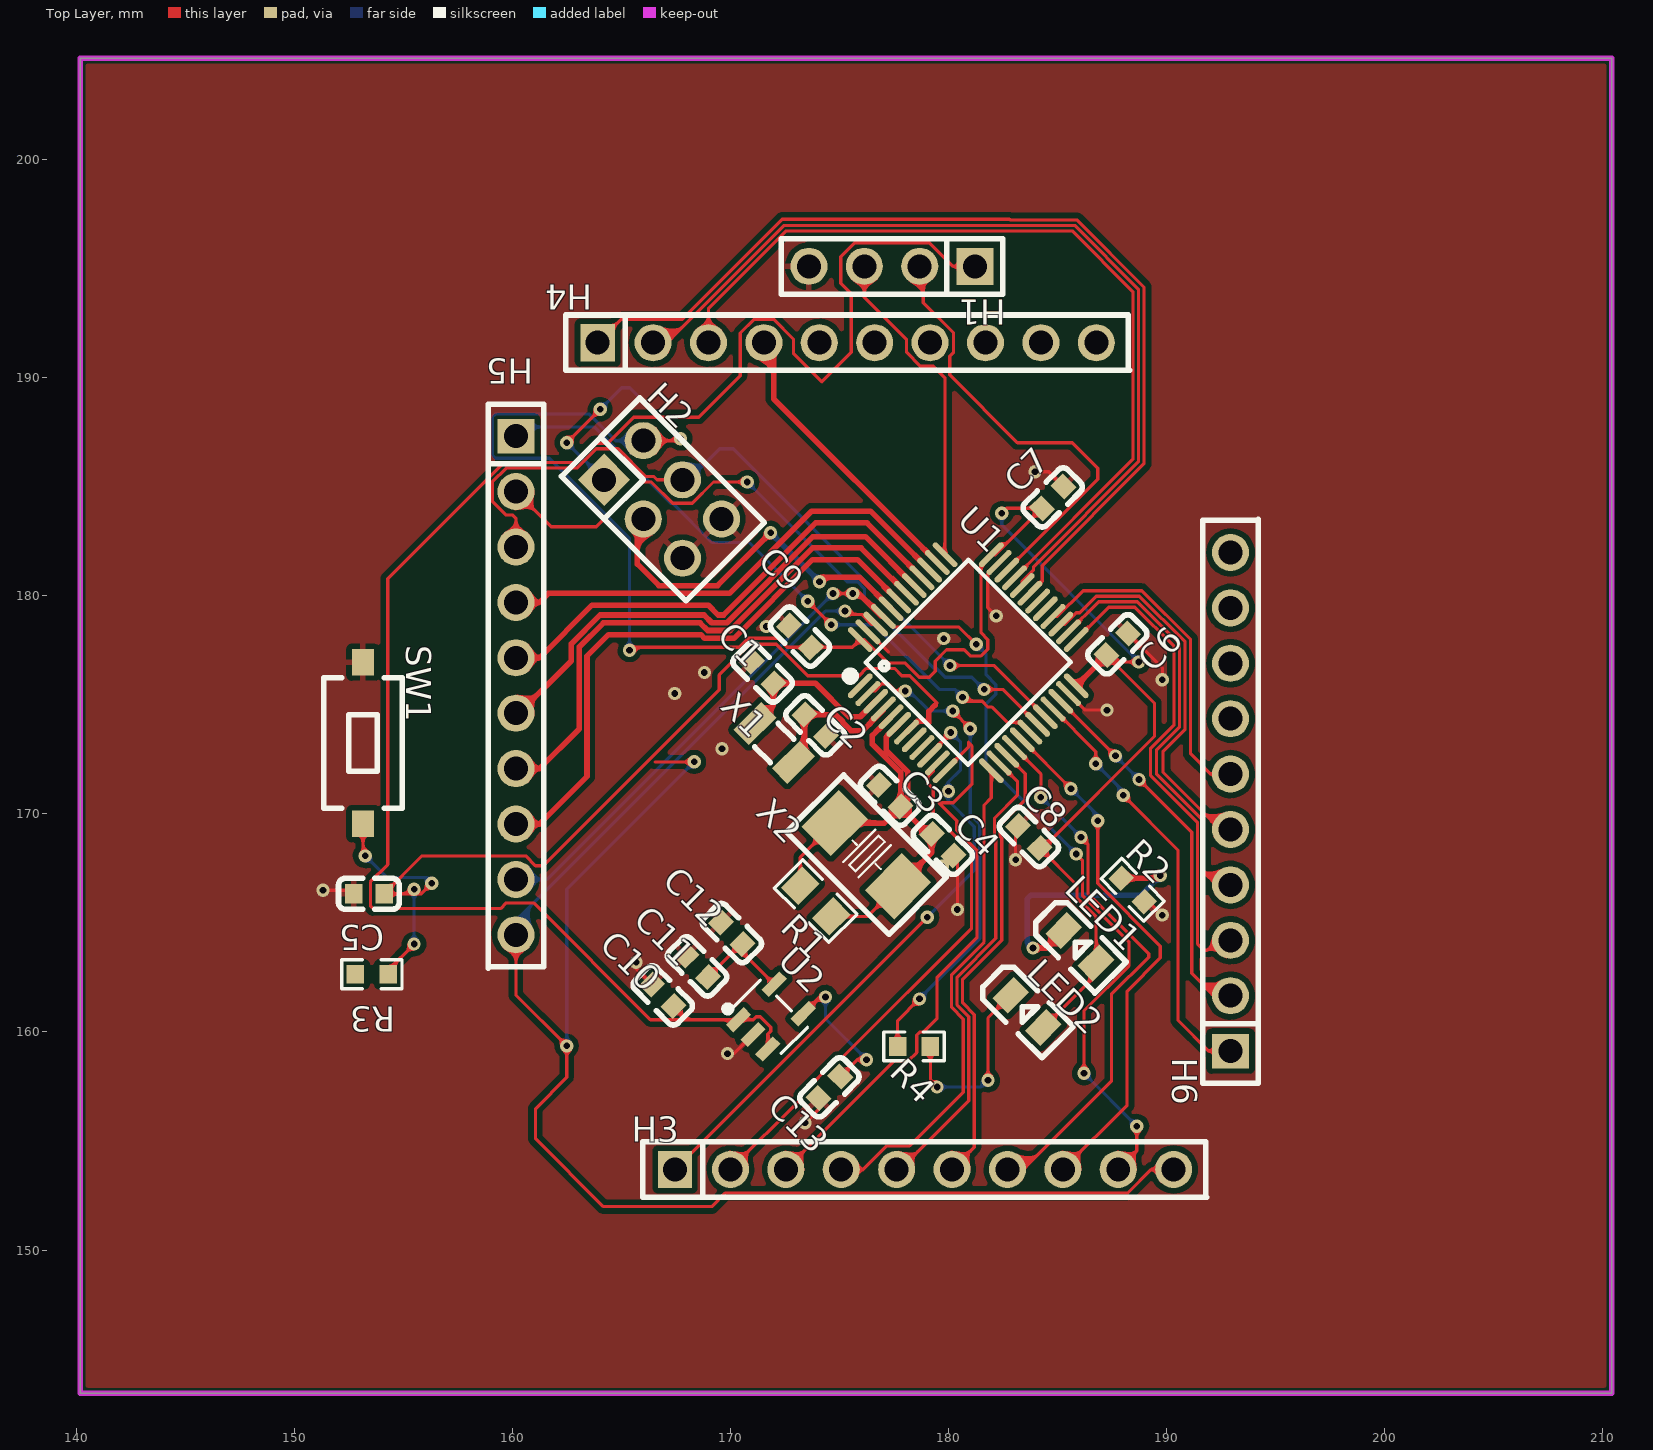
[diagram p0: Top Layer view]
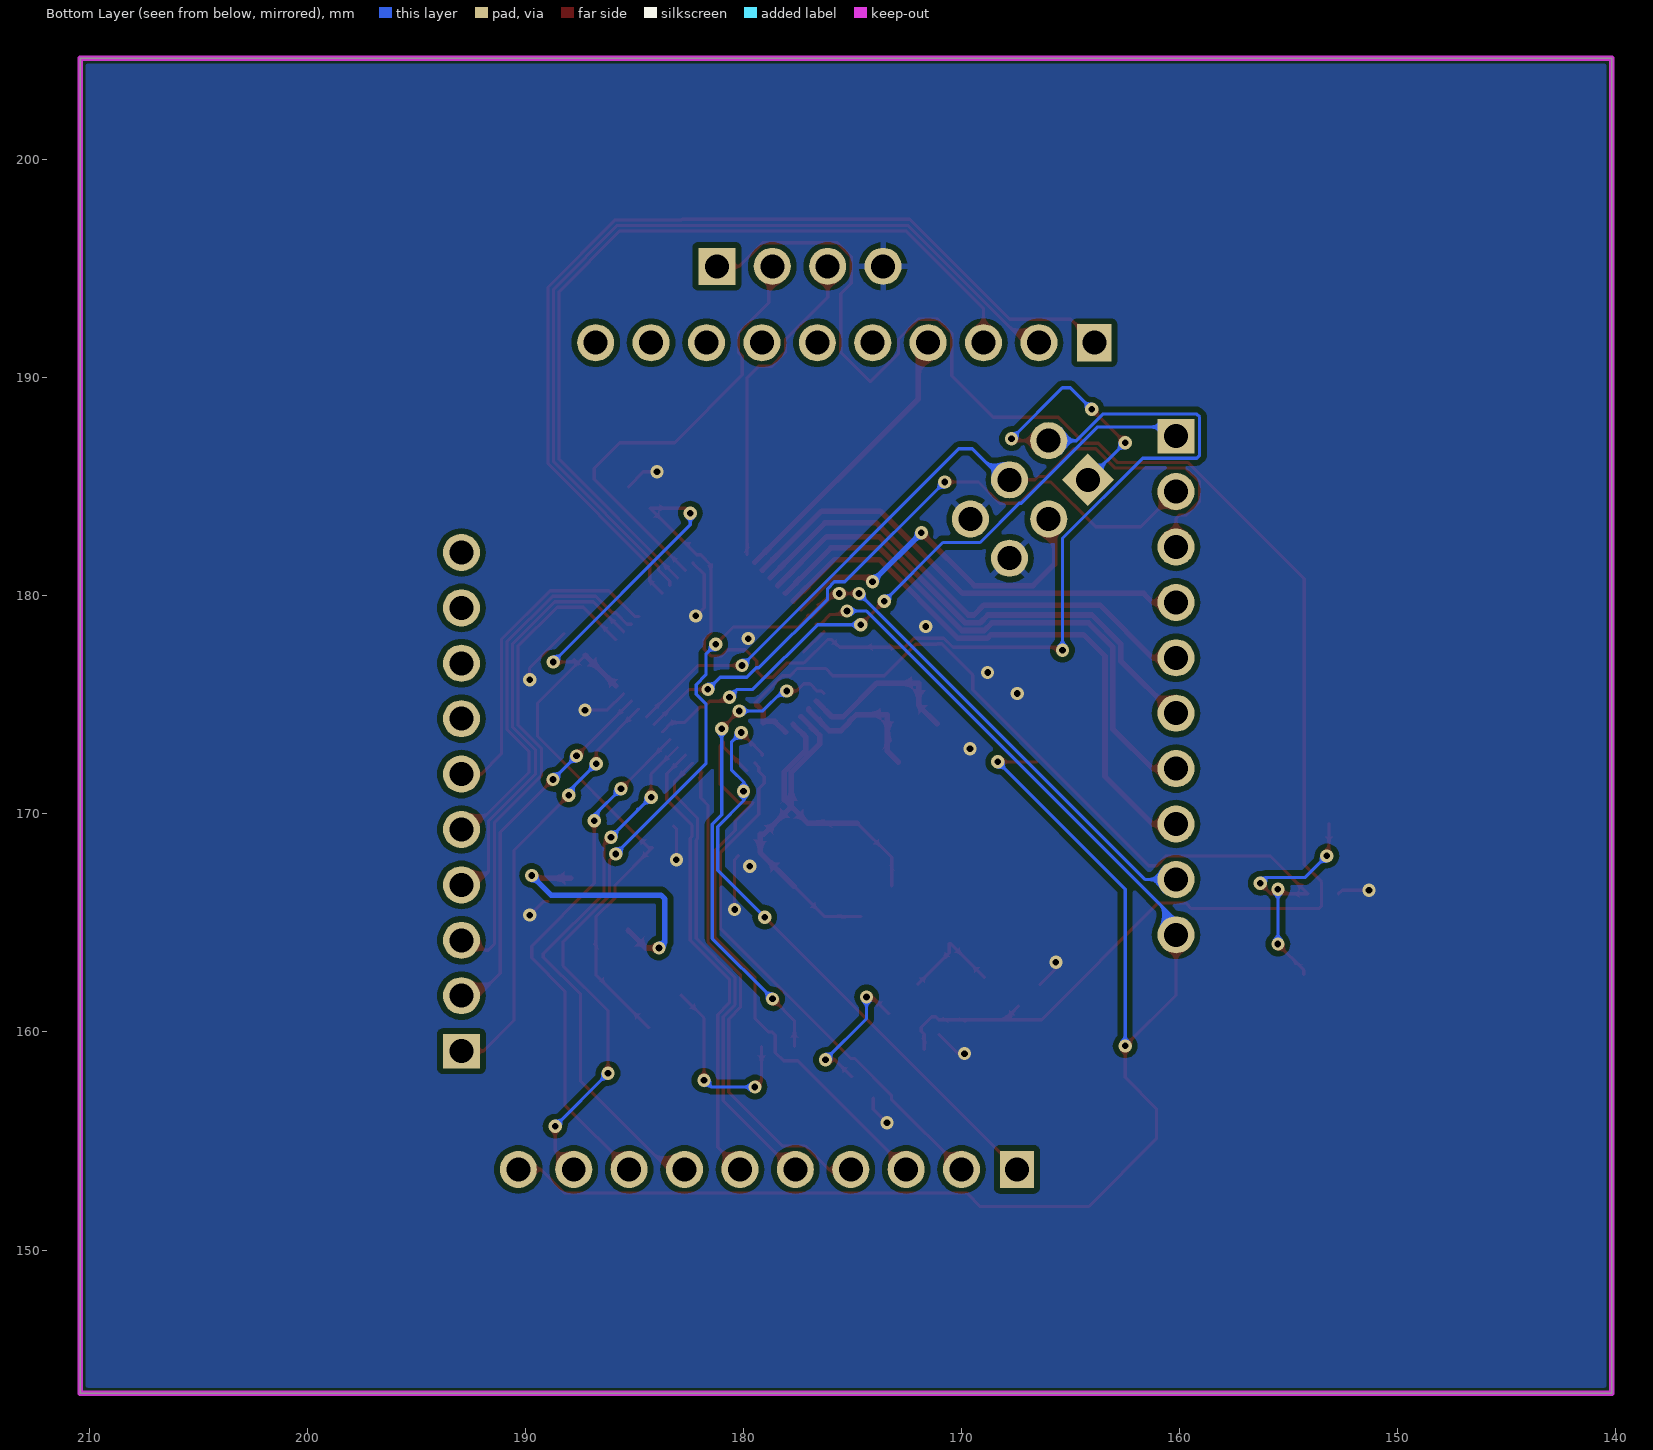
[diagram p1: Bottom Layer view, seen from below]
# Altium PCB MISC52025.pcbdoc
Units mm, origin at the board's own origin, x right, y up, seen from the top; angles counter-clockwise.
Board outline 70.23 x 61.21 mm, 2 copper layers (Top Layer, Bottom Layer), stack 1.58 mm thick; 30 components, 46 nets, 147 pads, 65 vias.

## Layer stack, top to bottom
Top Solder Mask Layer: solder mask 0.01, Dk 3.3
Top Layer: signal copper 0.035
Dielectric1: surface 1.51, FR4, Dk 4.5
Bottom Layer: signal copper 0.035
Bottom Solder Mask Layer: solder mask 0.01, Dk 3.3

## Board outline
140.182,204.647 140.182,143.433 210.413,143.433 210.413,204.647

## Design rules (kind name [scope] priority, off if disabled: settings)
BoardOutlineClearance copperThickness2oz_1 [All] p2 off: genericclearance=0.203 ignorepadtopadclearanceinfootprint=FALSE except(0: Arc-SplitContinuation Track-SplitContinuation SMDPad-SplitContinuation THPad-SplitContinuation Via-SplitContinuation Fill-SplitContinuation Region-SplitContinuation Poly-SplitContinuation Text-SplitContinuation Hole-SplitContinuation; 0.152: Arc-CutoutEdge SMDPad-CutoutEdge THPad-CutoutEdge Via-CutoutEdge Fill-CutoutEdge Region-CutoutEdge Text-CutoutEdge; 0.176: Hole-OutlineEdge Hole-CutoutEdge; 0.254: Poly-OutlineEdge Poly-CutoutEdge; 0.3: Arc-OutlineEdge Track-OutlineEdge SMDPad-OutlineEdge THPad-OutlineEdge Via-OutlineEdge Fill-OutlineEdge Region-OutlineEdge Text-OutlineEdge Track-CutoutEdge)
BoardOutlineClearance copperThickness1oz_1 [All] p4: genericclearance=0.102 ignorepadtopadclearanceinfootprint=FALSE except(0: Arc-SplitContinuation Track-SplitContinuation SMDPad-SplitContinuation THPad-SplitContinuation Via-SplitContinuation Fill-SplitContinuation Region-SplitContinuation Poly-SplitContinuation Text-SplitContinuation Hole-SplitContinuation; 0.152: SMDPad-CutoutEdge THPad-CutoutEdge Via-CutoutEdge Fill-CutoutEdge Region-CutoutEdge Text-CutoutEdge; 0.176: Hole-OutlineEdge Hole-CutoutEdge; 0.254: Poly-OutlineEdge Poly-CutoutEdge; 0.3: Arc-OutlineEdge Track-OutlineEdge SMDPad-OutlineEdge THPad-OutlineEdge Via-OutlineEdge Fill-OutlineEdge Region-OutlineEdge Text-OutlineEdge Arc-CutoutEdge Track-CutoutEdge)
Clearance copperThickness2oz [All] p1 off: gap=0.203 ignorepadtopadclearanceinfootprint=FALSE except(0.152: SMDPad-Track SMDPad-SMDPad THPad-Track SMDPad-THPad THPad-THPad Track-Via SMDPad-Via THPad-Via Via-Via Fill-Track Region-Track Fill-SMDPad Region-SMDPad Fill-THPad Region-THPad Fill-Via Region-Via Fill-Fill Fill-Region Region-Region Arc-Track Arc-SMDPad Arc-THPad Arc-Via Fill-Arc Region-Arc Arc-Arc Text-Track SMDPad-Text Text-THPad Text-Via Fill-Text Region-Text Arc-Text Text-Text; 0.176: Hole-Track Hole-SMDPad Hole-THPad Hole-Via Fill-Hole Region-Hole Hole-Arc Hole-Text; 0.254: Poly-Track Poly-SMDPad Poly-THPad Poly-Via Poly-Fill Poly-Region Poly-Poly Poly-Arc Poly-Text Poly-Hole)
Clearance copperThickness1oz [All] p3: gap=0.102 ignorepadtopadclearanceinfootprint=FALSE except(0.152: SMDPad-Track SMDPad-SMDPad THPad-Track SMDPad-THPad THPad-THPad Track-Via SMDPad-Via THPad-Via Via-Via Fill-Track Region-Track Fill-SMDPad Region-SMDPad Fill-THPad Region-THPad Fill-Via Region-Via Fill-Fill Fill-Region Region-Region Arc-Track Arc-SMDPad Arc-THPad Arc-Via Fill-Arc Region-Arc Arc-Arc Text-Track SMDPad-Text Text-THPad Text-Via Fill-Text Region-Text Arc-Text Text-Text; 0.176: Hole-Track Hole-SMDPad Hole-THPad Hole-Via Fill-Hole Region-Hole Hole-Arc Hole-Text; 0.254: Poly-Track Poly-SMDPad Poly-THPad Poly-Via Poly-Fill Poly-Region Poly-Poly Poly-Arc Poly-Text Poly-Hole)
DiffPairsRouting differentialPair [All] p1: maxlimit=0.152 minlimit=0.152 mostfreqgap=0.152 toplayer_minwidth=0.127 toplayer_prefwidth=0.254 toplayer_maxwidth=2.54 toplayer_mingap=0.152 toplayer_prefgap=0.152 toplayer_maxgap=0.152 bottomlayer_minwidth=0.127 bottomlayer_prefwidth=0.254 bottomlayer_maxwidth=2.54 bottomlayer_mingap=0.152 bottomlayer_prefgap=0.152 bottomlayer_maxgap=0.152 maxuncoupledlength=0.254
HoleToHoleClearance otherClearance [All] p1: gap=0.3 allowstackedmicrovias=TRUE
Length netLength [All] p1: minlimit=0 maxlimit=0
MatchedLengths netLengthTolerance [All] p1: tolerance=25.4
PasteMaskExpansion pasteMaskExpansion [All] p1: expansion=0
PlaneConnect innerPlane [All] p1: planeconnectstyle=Relief reliefexpansion=0.508 reliefentries=4 reliefconductorwidth=0.254 reliefairgap=0.254
PolygonConnect copperRegion [(InNet('GND'))] p1: connectstyle=Relief reliefconductorwidth=0.254 reliefentries=4 polygonreliefangle="90 Angle" airgapwidth=0.254 via.connectstyle=Relief via.reliefconductorwidth=0.254 via.reliefentries=4 via.polygonreliefangle="90 Angle" via.airgapwidth=0.254
RoutingVias viaSize [All] p1: holewidth=0.305 width=0.61 viastyle="Through Hole" minholewidth=0.3 minwidth=0.5 maxholewidth=6.3 maxwidth=10
SolderMaskExpansion solderMaskExpansion [IsVia] p1: expansion=-25.4 istentingtop=TRUE
SolderMaskExpansion solderMaskExpansion [All] p2: expansion=0.051 istentingtop=FALSE
Width copperThickness2oz_2 [All] p1 off: maxlimit=2.54 minlimit=0.203 preferedwidth=0.254
Width copperThickness1oz_2 [All] p2: maxlimit=2.54 minlimit=0.127 preferedwidth=0.254

## Components (designator, comment, footprint, x,y, rotation, side; value= is the part's Value field where it differs from the comment)
C1 "22pF" C0603 171.471,176.478 r315 top
C2 "22pF" C0603 173.895,174.053 r135 top
C3 "22pF" C0603 177.308,170.82 r315 top
C4 "22pF" C0603 179.733,168.575 r135 top
C5 "100nF" C0603 153.421,166.33 r0 top
C6 "100nF" C0603 187.735,177.767 r225 top
C7 "100nF" C0603 184.771,184.502 r225 top
C8 "100nF" C0603 183.684,168.934 r315 top
C9 "100nF" C0603 173.187,178.126 r315 top
C10 "10uF" C0603 166.901,161.672 r315 top
C11 "100nF" C0603 168.468,163.001 r315 top
C12 "1uF" C0603 170.066,164.53 r315 top
C13 "22nF" C0603 174.538,157.457 r45 top
H1 "PZ254V-11-04P" HDR-TH_4P-P2.54-V-M 177.407,195.099 r180 top
H2 "PZ254V-12-6P" HDR-TH_6P-P2.54-V-M-R2-C3-S2.54 166.901,184.412 r315 top
H3 "PH2.54-1X10P-H25" HDR-TH_10P-P2.54-V-M 178.889,153.695 r0 top
H4 "PH2.54-1X10P-H25" HDR-TH_10P-P2.54-V-M 175.342,191.596 r0 top
H5 "PH2.54-1X10P-H25" HDR-TH_10P-P2.54-V-M 160.165,175.881 r270 top
H6 "PH2.54-1X10P-H25" HDR-TH_10P-P2.54-V-M 192.929,170.55 r90 top
LED1 "HL-PSC-2012H233W(6000-7000K)" LED0805-R-RD 186.019,163.905 r315 top
LED2 "HL-PSC-2012H233W(6000-7000K)" LED0805-R-RD 183.594,160.942 r315 top
R1 "1MΩ" R0805 173.909,165.999 r315 top
R2 "510Ω" R0603 188.444,166.51 r315 top
R3 "10kΩ" R0603 153.558,162.641 r180 top
R4 "510Ω" R0603 178.414,159.332 r180 top
SW1 "TS-1101-C-W" SW-SMD_L6.0-W3.3-LS8.0_TS-1101-C-W 153.151,173.245 r270 top
U1 "STM32F103C8T6" LQFP-48_L7.0-W7.0-P0.50-LS9.0-BL 180.9,176.927 r315 top
U2 "RT9193-33GB" SOT-23-5_L3.0-W1.7-P0.95-LS2.8-BL 171.853,160.698 r315 top
X1 "32.768kHz" FC-135R_L3.2-W1.5 172.01,173.245 r135 top
X2 "8MHz" CRYSTAL-SMD_L5.0-W3.2 176.23,168.126 r135 top

## Footprints (in the part's own frame and the unit in brackets; to place one, negate y for a bottom-side part, rotate by r counter-clockwise, add the part's x,y. Pads: shape width x height; smd on the part's side, far side on the other; paste and mask are expansions set on the pad)
C0603 [mm]
  rect 0.8x0.9 smd: 1(-0.7,0) 2(0.7,0)
  silkscreen extent -1.39,-0.71 1.39,0.71
CRYSTAL-SMD_L5.0-W3.2 [mm]
  rect 1.9x2.4 smd: 1(-2.05,0) 2(2.05,0)
  silkscreen extent -3.32,-1.85 3.33,1.85
FC-135R_L3.2-W1.5 [mm]
  rect 1x1.8 smd: 1(-1.25,0) 2(1.25,0)
  silkscreen extent -0.51,-0.76 0.51,0.76
HDR-TH_4P-P2.54-V-M [mm]
  rect 1.7x1.7 hole 1.1: 1(-3.81,0)
  round 1.7 hole 1.1: 2(-1.27,0) 3(1.27,0) 4(3.81,0)
  silkscreen extent -5.08,-1.27 5.08,1.27
HDR-TH_6P-P2.54-V-M-R2-C3-S2.54 [mm]
  rect 1.7x1.7 hole 1.1: 1(-2.54,-1.27)
  round 1.7 hole 1.1: 2(-2.54,1.27) 3(0,-1.27) 4(0,1.27) 5(2.54,-1.27) 6(2.54,1.27)
  silkscreen extent -4.04,-2.54 4.04,2.54
HDR-TH_10P-P2.54-V-M [mm]
  rect 1.575x1.7 hole 1.1: 1(-11.43,0)
  round 1.7 hole 1.1: 2(-8.89,0) 3(-6.35,0) 4(-3.81,0) 5(-1.27,0) 6(1.27,0) 7(3.81,0) 8(6.35,0) 9(8.89,0) 10(11.43,0)
  silkscreen extent -12.9,-1.27 12.95,1.27
LED0805-R-RD [mm]
  rect 1x1.4 smd: 1(1.05,0) 2(-1.05,0)
  silkscreen extent -2.22,-1.04 1.99,1.01
LQFP-48_L7.0-W7.0-P0.50-LS9.0-BL [mm]
  oval 0.27x1.5 smd paste+0 mask+0.05: 1(-2.75,-4.25) 2(-2.25,-4.25) 3(-1.75,-4.25) 4(-1.25,-4.25) 5(-0.75,-4.25) 6(-0.25,-4.25) 7(0.25,-4.25) 8(0.75,-4.25) 9(1.25,-4.25) 10(1.75,-4.25) 11(2.25,-4.25) 12(2.75,-4.25) 25(2.75,4.25) 26(2.25,4.25) 27(1.75,4.25) 28(1.25,4.25) 29(0.75,4.25) 30(0.25,4.25) 31(-0.25,4.25) 32(-0.75,4.25) 33(-1.25,4.25) 34(-1.75,4.25) 35(-2.25,4.25) 36(-2.75,4.25)
  oval 1.5x0.27 smd paste+0 mask+0.05: 13(4.25,-2.75) 14(4.25,-2.25) 15(4.25,-1.75) 16(4.25,-1.25) 17(4.25,-0.75) 18(4.25,-0.25) 19(4.25,0.25) 20(4.25,0.75) 21(4.25,1.25) 22(4.25,1.75) 23(4.25,2.25) 24(4.25,2.75) 37(-4.25,2.75) 38(-4.25,2.25) 39(-4.25,1.75) 40(-4.25,1.25) 41(-4.25,0.75) 42(-4.25,0.25) 43(-4.25,-0.25) 44(-4.25,-0.75) 45(-4.25,-1.25) 46(-4.25,-1.75) 47(-4.25,-2.25) 48(-4.25,-2.75)
  silkscreen extent -3.59,-4.46 3.3,3.34
R0603 [mm]
  rect 0.806x0.864 smd paste-100 mask+0.051: 1(-0.753,0) 2(0.753,0)
  silkscreen extent -1.39,-0.66 1.39,0.66
R0805 [mm]
  rect 1.133x1.377 smd paste-100 mask+0.051: 1(-1,0) 2(1,0)
  silkscreen extent -1.76,-0.92 1.76,0.92
SOT-23-5_L3.0-W1.7-P0.95-LS2.8-BL [mm]
  rect 0.49x1.157 smd: 1(-0.95,-1.154) 2(0,-1.154) 3(0.95,-1.154)
  rect 0.49x1.175 smd: 4(0.95,1.154) 5(-0.95,1.154)
  silkscreen extent -1.8,-1.29 1.53,0.85
SW-SMD_L6.0-W3.3-LS8.0_TS-1101-C-W [mm]
  rect 1.2x1 smd: 1(-3.7,0) 2(3.7,0)
  silkscreen extent -3,-1.8 3,1.8

## Via types
v1: diameter 0.61, hole 0.305, Top Layer to Bottom Layer, 65 vias

## Nets (pads, with @x,y where several pads share a name; then routed paths per layer and width w, separated by ;. In a path a pad name is that pad's centre, name@x,y a point inside that pad or via, vN(x,y) a via of type N, cw(c..) or ccw(c..) an arc to the next point about the centre after c; other vN are vias at no path point)
$1N2: LED1.2 R2.1 | length 12.5
  Top Layer w0.254: v1(183.873,163.847) 184.475,163.847 LED1.2 ; R2.1 189.583,167.042 v1(189.71,167.17)
  Bottom Layer w0.254: v1(183.873,163.847) 183.604,164.117 183.604,166.092 183.783,166.272 188.812,166.272 v1(189.71,167.17)
$1N4: LED2.2 R4.1 | length 8.8
  Top Layer w0.15: R4.1 179.168,157.776 v1(179.473,157.471) ; v1(181.808,157.778) 181.808,160.641 LED2.2
  Bottom Layer w0.15: v1(179.473,157.471) 181.449,157.471 181.755,157.778 v1(181.808,157.778)
$1N5: R4.2 U1.2 | length 22
  Top Layer w0.15: U1.2 176.419,175.628 176.614,175.628 176.942,175.956 177.242,175.956 177.571,175.628 v1(178.02,175.628) ; R4.2 177.661,160.509 v1(178.665,161.512) ; v1(180.191,174.713) v1(181,173.905)
  Bottom Layer w0.15: v1(178.02,175.628) 178.051,175.597 178.231,175.597 179.114,174.713 v1(180.191,174.713) ; v1(178.665,161.512) 181.431,164.279 181.431,169.519 181,169.951 v1(181,173.905)
$1N7: C1.2 U1.3 X1.2 | length 7.8
  Top Layer w0.254: X1.2 171.966,174.969 C1.2 173.893,175.983 175.432,174.444 175.942,174.444 U1.3
$1N12: C3.2 C4.2 R1.1 R1.2 U1.5 U1.6 X2.1 X2.2 | length 25.1
  Top Layer w0.15: R1.1 173.202,167.997 X2.2 ; R1.2 176.295,165.292 X2.1
  Top Layer w0.254: X2.2 177.053,169.576 C3.2 ; U1.5 176.509,173.597 176.509,173.187 177.803,171.893 C3.2 ; X2.1 179.238,168.234 C4.2 179.058,169.07 C3.2 ; U1.6 177.138,173.518 177.138,172.917 178.126,171.93 178.126,170.648 C3.2
$1N13: C2.2 U1.4 X1.1 | length 6.8
  Top Layer w0.254: X1.1 173.401,172.868 C2.2 174.824,174.548 175.147,174.225 175.147,174.19 175.522,173.815 176.075,173.815 177.011,174.751 U1.4
$1N15: C5.2 R3.1 SW1.2 U1.7 | length 46.6
  Top Layer w0.15: SW1.2 153.151,168.168 v1(153.251,168.068) ; R3.1 154.312,162.843 v1(155.496,164.027) ; v1(155.496,166.541) v1@155.284,166.33 ; v1(156.304,166.811) 155.823,166.33 v1@155.284,166.33 ; 179.473,175.073 178.216,176.33 177.854,176.33 177.52,176.663 176.235,176.663 175.902,176.33 173.546,176.33 172.109,177.767 171.139,177.767 171.105,177.801 170.917,177.801 169.483,176.367 169.483,175.679 161.423,167.619 161.06,167.619 160.611,168.068 155.858,168.068 C5.2 v1@155.284,166.33
  Top Layer w0.254: U1.7 178.567,174.24 179.032,174.24 179.097,174.175 179.097,174.697 179.383,174.983
  Bottom Layer w0.15: v1(153.251,168.068) 154.238,167.08 156.034,167.08 v1(156.304,166.811) ; v1(155.496,164.027) v1(155.496,166.541)
$1N18: H1.2 U1.34 | length 20.7
  Top Layer w0.15: H1.2 178.844,194.932 178.844,193.427 180.229,192.042 180.229,191.15 180.049,190.97 180.049,190.122 183.155,187.016 185.669,187.016 186.837,185.849 186.837,185.338 U1.34
$1N19: H1.3 U1.37 | length 15.1
  Top Layer w0.15: H1.3 176.137,193.675 178.075,191.737 178.075,191.15 178.706,190.519 179.293,190.519 179.84,189.972 U1.37
$1N32: C13.2 U2.4 | length 6.5
  Top Layer w0.15: U2.4 174.101,161.602 v1(174.354,161.602) ; C13.2 175.809,158.729 v1(176.24,158.729)
  Bottom Layer w0.15: v1(174.354,161.602) 174.354,160.614 v1(176.24,158.729)
+3,3V: R3.2
+3.3V: C6.2 C7.2 C8.2 C9.2 H2.1 H2.2 LED1.1 LED2.1 U1.24 U1.36 U1.48 | length 97
  Top Layer w0.15: v1(162.5,187.016) v1(164.027,188.543) ; v1(165.374,177.497) 165.508,177.631 170.391,177.631 170.813,178.053 172.179,178.053 172.601,177.631 C9.2 175.594,177.631 U1.48 176.146,177.987 177.218,176.915 177.993,176.915 178.65,176.257 179.115,176.257 179.389,176.531 179.389,177 179.904,177.515 180.71,177.515 180.99,177.235 181.489,177.235 181.801,177.546 181.801,177.987 181.489,178.299 181.489,181.405 U1.36 182.146,181.877 C7.2 182.66,184.007 v1(182.436,183.783) ; H2.2 167.619,187.106 v1(167.709,187.196) ; LED2.1 186.762,162.624 LED1.1 186.762,165.275 185.884,166.153 185.884,166.735 C8.2 184.334,168.439 189.441,173.546 189.441,175.07 C6.2@187.553,176.958 ; C6.2 C6.2@187.553,176.958 ; v1(188.723,176.958) C6.2@187.553,176.958
  Top Layer w0.254: U1.24 187.24,177.256 C6.2
  Bottom Layer w0.15: v1(162.5,187.016) H2.1 ; v1(164.027,188.543) 165.015,189.531 165.374,189.531 v1(167.709,187.196) ; v1(165.374,177.497) 165.374,182.62 161.697,186.296 159.221,186.296 159.088,186.429 159.088,188.192 159.221,188.325 163.526,188.325 164.745,187.106 H2.2 ; v1(182.436,183.783) 182.436,183.245 v1(188.723,176.958)
+5V: C10.2 H1.1 U2.1 U2.3 | length 79.2
  Top Layer w0.15: C10.2 168.019,160.554 ; U2.3 171.709,159.886 171.847,160.024 171.847,160.212 171.367,160.692 171.179,160.692 171.042,160.554 U2.1 168.019,160.554 ; H1.1 180.201,195.099 179.124,196.176 175.691,196.176 175.06,195.545 175.06,194.318 175.535,193.843 175.535,191.15 174.192,189.807 172.885,191.114 172.885,191.766 171.978,192.673 171.086,192.673 170.455,192.042 170.455,190.087 168.552,188.183 165.556,188.183 164.364,186.991 163.735,186.991 162.844,186.1 159.615,186.1 154.291,180.776 154.291,167.671 153.494,166.874 153.494,165.786 153.627,165.653 159.459,165.653 159.719,165.914 160.973,165.914 166.332,160.554 168.019,160.554
BOOT0: H2.3 U1.44 | length 16.8
  Top Layer w0.254: H2.3 165.733,183.245 165.733,181.449 166.721,180.461 169.415,180.461 v1(171.84,182.885) ; v1(174.085,180.64) 174.297,180.853 175.913,180.853 U1.44
  Bottom Layer w0.254: v1(171.84,182.885) v1(174.085,180.64)
GND: C1.1 C2.1 C3.1 C4.1 C5.1 C6.1 C7.1 C8.1 C9.1 C10.1 C11.1 C12.1 C13.1 H1.4 H2.5 H2.6 R2.2 SW1.1 U1.23 U1.35 U1.47 U2.2 | length 21.5
  Top Layer w0.15: v1(151.322,166.498) 152.552,166.498 C5.1 ; v1(165.673,163.196) 165.673,162.9 C10.1 ; v1(169.864,159.005) 170.161,159.005 U2.2 ; v1(173.42,155.83) 174.043,156.454 C13.1 ; U1.47 177.225,177.42 177.23,177.42 ; C4.1 180.405,167.903 v1(180.405,165.609) ; v1(182.183,179.071) 181.802,179.452 181.802,180.976 182.314,181.489 U1.35 ; v1(183.072,167.895) 183.072,169.312 C8.1 ; v1(183.961,185.675) 184.588,185.675 C7.1 ; U1.23 186.255,174.753 v1(187.263,174.753) ; C6.1 189.803,176.688 v1(189.803,176.15) ; R2.2 189.181,165.977 v1(189.803,165.355)
  other v1: 179.712,167.592 169.61,172.975 167.451,175.515 168.806,176.478 179.778,178.031 171.642,178.585
PA0: H3.1 U1.10 | length 28.1
  Top Layer w0.15: H3.1 v1(179.023,165.259) ; U1.10 179.132,172.756 v1(180.102,173.726)
  Bottom Layer w0.15: v1(179.023,165.259) 181.179,167.415 181.179,169.415 179.974,170.62 v1@179.974,171.032 ; v1(179.995,171.032) v1@179.974,171.032 ; v1(180.102,173.726) 180.551,173.277 180.551,172.019 179.974,171.443 v1@179.974,171.032
PA1: H3.2 U1.11 | length 24.3
  Top Layer w0.15: H3.2 173.215,156.912 173.215,157.092 174.904,158.781 175.084,158.781 181.056,164.752 181.056,168.21 179.293,169.972 179.293,171.142 179.043,171.392 179.043,171.692 179.293,171.943 179.293,172.138 U1.11
PA2: H3.3 U1.12 | length 27.2
  Top Layer w0.15: H3.3 177.516,158.673 178.158,158.673 178.538,159.052 178.538,159.858 178.671,159.991 178.834,159.991 179.473,160.629 179.473,162.5 181.308,164.335 181.308,168.314 180.371,169.251 180.371,169.684 179.563,170.493 179.57,170.5 180.216,170.5 181.072,171.356 181.072,173.112 180.91,173.274 180.91,173.047 U1.12
PA3: H3.4 U1.13 | length 22.8
  Top Layer w0.15: H3.4 176.096,153.695 177.173,154.772 178.21,154.772 180.675,157.237 180.675,160.585 180.136,161.124 180.136,162.625 181.628,164.117 181.628,170.403 181.961,170.735 U1.13
PA4: H3.5 U1.14 | length 21.9
  Top Layer w0.15: H3.5 177.784,153.695 180.927,156.839 180.927,160.69 180.388,161.228 180.388,162.515 182.167,164.293 182.167,168.789 182.109,168.847 182.109,169.806 183.155,170.852 183.155,171.49 U1.14
PA5: H3.6 U1.15 | length 21.2
  Top Layer w0.15: H3.6 181.179,154.715 181.179,160.794 180.64,161.333 180.64,162.41 182.436,164.207 182.436,168.876 182.361,168.952 182.361,169.488 183.514,170.641 183.514,171.838 U1.15
PA6: H3.7 U1.16 | length 25.1
  Top Layer w0.15: H3.7 183.42,153.695 187.465,157.741 187.465,161.722 189.172,163.428 189.172,163.578 186.388,166.362 186.388,168.607 v1(186.073,168.921) ; U1.16 184.232,171.827 v1(184.232,170.762)
  Bottom Layer w0.15: v1(184.232,170.762) 184.771,170.223 ; 184.861,170.223 184.771,170.223 ; v1(186.073,168.921) 184.771,170.223
PA7: H3.8 U1.17 | length 24.2
  Top Layer w0.15: U1.17 v1(185.612,171.154) ; H3.8 188.184,156.64 188.184,161.872 189.71,163.398 189.71,163.937 186.837,166.811 v1(186.837,169.684)
  Bottom Layer w0.15: v1(185.612,171.154) 186.837,169.929 v1(186.837,169.684)
PA8: U1.29
PA9: U1.30
PA10: H4.1 U1.31 | length 44.9
  Top Layer w0.15: H4.1 164.99,192.674 167.799,192.674 172.379,197.254 182.796,197.254 182.825,197.224 185.883,197.224 188.957,194.151 188.957,186.039 184.3,181.381 184.3,180.68 U1.31
PA11: H4.2 U1.32 | length 41.5
  Top Layer w0.15: H4.2 167.08,191.596 168.427,192.943 168.43,192.943 172.459,196.972 185.779,196.972 188.705,194.046 188.705,186.143 183.895,181.333 183.895,181.178 183.375,180.657 U1.32
PA12: H4.3 U1.33 | length 39
  Top Layer w0.15: H4.3 168.992,193.149 172.563,196.72 185.675,196.72 188.453,193.942 188.453,186.248 U1.33
PA15: H4.4 U1.38 | length 13.4
  Top Layer w0.254: H4.4 171.981,191.147 171.981,189.028 U1.38
PB0: H5.1 U1.18 | length 29.5
  Top Layer w0.15: v1(173.546,179.742) v1(174.624,178.665) ; v1(180.64,175.342) 180.82,175.162 181.538,175.162 181.808,174.893 181.994,174.893 182.699,174.188 183.285,174.188 U1.18
  Bottom Layer w0.15: H5.1 160.589,187.735 163.757,187.735 167.26,184.232 167.353,184.232 169.149,182.437 170.851,182.437 v1(173.546,179.742) ; v1(174.624,178.665) 176.599,178.665 179.563,175.701 180.281,175.701 v1(180.64,175.342)
PB1: H5.2 U1.19 | length 31.1
  Top Layer w0.15: H5.2 161.781,183.155 163.847,183.155 165.904,185.211 166.374,185.211 167.353,184.233 168.245,184.233 169.223,185.211 v1(170.771,185.211) ; v1(181.628,175.701) 182.479,175.701 U1.19
  Bottom Layer w0.15: v1(170.771,185.211) 175.349,180.634 175.832,180.634 176.143,180.322 176.143,179.839 179.293,176.689 179.419,176.689 179.845,176.263 181.067,176.263 v1(181.628,175.701)
PB2: H2.4 H5.3 U1.20 | length 35.9
  Top Layer w0.15: H5.3 160.165,183.548 160.02,183.694 159.719,183.694 159.088,184.325 159.088,185.217 159.719,185.848 162.948,185.848 163.84,186.739 164.846,186.739 166.122,185.463 166.479,185.463 166.632,185.31 H2.4 ; v1(180.065,176.795) 182.093,176.795 U1.20
  Bottom Layer w0.15: H2.4 168.078,185.31 169.505,186.737 170.123,186.737 v1(180.065,176.795)
PB3: H5.4 U1.39 | length 21.8
  Top Layer w0.254: H5.4 161.243,179.691 161.654,180.102 169.954,180.102 173.726,183.873 176.42,183.873 179.124,181.169 U1.39
PB4: H5.5 U1.40 | length 22.6
  Top Layer w0.254: H5.5 161.243,177.151 163.655,179.563 168.981,179.563 169.43,179.114 169.684,179.114 173.905,183.334 176.26,183.334 U1.40
PB5: H5.6 U1.41 | length 23.3
  Top Layer w0.254: H5.6 160.3,174.611 162.7,177.011 162.7,177.786 164.027,179.114 168.786,179.114 169.142,178.758 169.832,178.758 173.78,182.706 176.182,182.706 U1.41
PB6: H5.7 U1.42 | length 25.5
  Top Layer w0.254: H5.7 161.243,172.071 163.066,173.894 163.066,177.65 164.171,178.755 168.607,178.755 168.96,178.402 169.979,178.402 173.766,182.188 175.992,182.188 U1.42
PB7: H5.8 U1.43 | length 26.7
  Top Layer w0.254: H5.8 161.243,169.531 163.422,171.71 163.422,177.228 164.41,178.216 168.642,178.216 168.812,178.046 170.158,178.046 173.768,181.655 175.818,181.655 U1.43
PB8: H3.9 H5.9 U1.45 | length 57.1
  Top Layer w0.15: v1(174.704,180.102) v1(175.611,180.102) ; U1.45 177.496,178.563 180.472,178.563 v1(181.269,177.767) ; v1(185.849,168.158) 186.136,167.871 186.136,166.257 188.274,164.12 188.274,163.039 186.208,160.974 v1(186.208,158.1) ; H3.9 188.633,154.549 v1(188.633,155.675)
  Top Layer w0.254: v1(175.611,180.102) 175.881,180.102 176.934,179.048 U1.45
  Bottom Layer w0.15: H5.9 161.594,166.991 v1(174.704,180.102) ; v1(181.269,177.767) 181.718,177.318 181.718,176.364 182.16,175.922 182.16,175.481 181.718,175.039 181.718,172.289 v1(185.849,168.158) ; v1(186.208,158.1) v1(188.633,155.675)
PB9: H3.10 H5.10 U1.46 | length 82.7
  Top Layer w0.15: H5.10 160.165,161.692 v1(162.5,159.357) 162.5,157.92 161.063,156.483 161.063,155.107 164.177,151.993 169.146,151.993 169.77,152.618 188.225,152.618 189.302,153.695 H3.10 ; 166.539,172.379 v1(168.337,172.379) ; v1(175.252,179.293) 175.408,179.138 176.019,179.138 176.462,178.694 U1.46
  Bottom Layer w0.15: H5.10 160.165,165.105 174.354,179.293 175.008,179.293 v1(175.252,179.293) ; v1(162.5,159.357) 162.5,166.541 v1(168.337,172.379)
PB10: H6.1 U1.21 | length 19.6
  Top Layer w0.15: U1.21 186.747,172.848 v1(186.747,172.289) ; v1(188.004,170.852) 190.519,168.337 190.519,160.525 191.923,159.12 H6.1
  Bottom Layer w0.15: v1(186.747,172.289) 188.004,171.032 v1(188.004,170.852)
PB11: H6.2 U1.22 | length 17.2
  Top Layer w0.15: U1.22 v1(187.649,172.652) ; v1(188.727,171.575) 191.147,169.155 191.147,162.68 192.167,161.66 H6.2
  Bottom Layer w0.15: v1(187.649,172.652) v1(188.727,171.575)
PB12: H6.3 U1.25 | length 22.7
  Top Layer w0.15: U1.25 187.335,179.473 188.543,179.473 190.339,177.677 190.339,174.085 189.261,173.007 189.261,171.75 191.417,169.595 191.417,164.027 191.701,163.743 191.851,163.743 191.882,163.774 192.503,163.774 H6.3
PB13: H6.4 U1.26 | length 19.7
  Top Layer w0.15: U1.26 186.88,179.725 188.647,179.725 190.591,177.781 190.591,173.98 189.531,172.92 189.531,171.84 191.686,169.684 191.686,167.35 192.296,166.74 H6.4
PB14: H6.5 U1.27 | length 17.7
  Top Layer w0.15: U1.27 185.338,178.694 185.858,179.215 186.014,179.215 186.776,179.977 188.752,179.977 190.843,177.886 190.843,173.876 189.835,172.868 189.835,171.892 192.447,169.28 H6.5
PB15: H6.6 U1.28 | length 15.2
  Top Layer w0.15: U1.28 184.984,179.048 186.165,180.229 188.856,180.229 191.095,177.99 191.095,172.742 192.017,171.82 H6.6
VCC: C11.2 C12.2 U2.5 | length 4.7
  Top Layer w0.15: C11.2 170.493,164.035 C12.2 170.561,163.622 U2.5
pads on no net: H4.5 H4.6 H4.7 H4.8 H4.9 H4.10 H6.7 H6.8 H6.9 H6.10 U1.1 U1.8 U1.9

## Polygon pours and split planes (outlines as drawn)
GND on Bottom Layer (solid, remove dead copper, pour order 2): 177.497,269.904 85.988,178.395 179.653,84.731 271.161,176.24
GND on Top Layer (solid, remove dead copper, pour order 0): 174.803,284.991 76.2,186.388 186.388,76.2 284.991,174.803

## Keep-outs
Board Outline Layer:
  the board outline again, w0.254

## Other copper
Top Layer:
  drawing of 165 lines, arcs and shapes, not listed
Bottom Layer:
  region net BOOT0: 173.701,180.844 173.881,181.024 173.92,180.997 173.977,180.973 174.042,180.954 174.104,180.945 173.78,180.621 173.771,180.684 173.752,180.749 173.728,180.806
  region net BOOT0: 172.223,182.682 172.044,182.502 172.005,182.528 171.948,182.553 171.883,182.572 171.821,182.581 172.144,182.905 172.154,182.842 172.172,182.777 172.197,182.72
  region net PB8: 174.464,179.755 174.358,179.861 174.371,179.893 174.383,179.954 174.4,180.121 174.723,179.797 174.557,179.78 174.496,179.768
  region net PB8: 161.323,167.066 161.323,166.916 161.278,166.911 161.234,166.896 161.19,166.873 161.147,166.843 161.104,166.807 161.062,166.766 160.982,166.675 160.907,166.579 160.839,166.487 160.779,166.409 160.728,166.353 160.728,167.628 160.779,167.573 160.839,167.495 160.907,167.403 160.982,167.306 161.062,167.215 161.104,167.174 161.147,167.138 161.19,167.108 161.234,167.086 161.278,167.071
  region net PB9: 174.837,179.218 174.837,179.368 174.869,179.382 174.921,179.416 175.05,179.522 175.05,179.065 174.921,179.17 174.869,179.205
  region net PB9: 160.295,165.34 160.891,165.724 160.863,165.688 160.84,165.645 160.823,165.595 160.811,165.54 160.803,165.481 160.8,165.419 160.804,165.289 160.82,165.16 160.845,165.041 160.875,164.94 160.906,164.867 159.659,165.134 159.682,165.147 159.711,165.159 159.78,165.176 159.954,165.204 160.048,165.222 160.14,165.248 160.183,165.265 160.224,165.286 160.261,165.311
  region net PB11: 187.996,172.412 187.89,172.306 187.858,172.319 187.797,172.331 187.63,172.348 187.954,172.672 187.971,172.505 187.983,172.444
  region net PB11: 188.38,171.815 188.486,171.921 188.519,171.908 188.58,171.896 188.746,171.879 188.423,171.556 188.406,171.722 188.394,171.783
  region net PB10: 187.094,172.048 186.988,171.942 186.955,171.956 186.894,171.967 186.728,171.984 187.051,172.308 187.068,172.141 187.08,172.08
  region net PB10: 187.693,171.237 187.934,171.208 187.959,171.188 187.987,171.172 188.048,171.15 188.106,171.135 188.148,171.121 187.719,170.961 187.73,170.997 187.737,171.036 187.739,171.075 187.737,171.115 187.731,171.152 187.722,171.186 187.709,171.215
  region net PB2: 179.719,177.035 179.825,177.141 179.857,177.128 179.918,177.116 180.085,177.099 179.761,176.776 179.744,176.942 179.732,177.003
  region net PB2: 168.798,186.136 168.694,185.82 168.666,185.785 168.644,185.745 168.628,185.7 168.616,185.651 168.609,185.599 168.606,185.544 168.606,185.432 168.619,185.218 168.621,185.129 168.618,185.092 168.611,185.061 167.944,186.148 168.125,186.11 168.244,186.087 168.371,186.067 168.498,186.058 168.559,186.058 168.617,186.062 168.671,186.072 168.719,186.087 168.762,186.108
  region net PB1: 181.282,175.942 181.388,176.048 181.42,176.034 181.481,176.023 181.647,176.006 181.324,175.682 181.307,175.849 181.295,175.91
  region net PB1: 171.118,184.971 171.012,184.865 170.98,184.878 170.918,184.89 170.752,184.907 171.075,185.23 171.092,185.064 171.104,185.003
  region net PB0: 180.294,175.583 180.4,175.689 180.432,175.675 180.493,175.663 180.659,175.646 180.336,175.323 180.319,175.489 180.307,175.55
  region net PB0: 175.039,178.74 175.039,178.59 175.007,178.577 174.955,178.542 174.825,178.436 174.825,178.893 174.955,178.788 175.007,178.753
  region net PB0: 173.199,179.983 173.305,180.089 173.338,180.076 173.399,180.064 173.565,180.047 173.242,179.723 173.225,179.89 173.213,179.951
  region net PB0: 161.24,187.81 161.24,187.66 161.176,187.652 161.115,187.63 161.06,187.594 161.015,187.547 161.015,187.922 161.06,187.875 161.115,187.839 161.176,187.817 161.24,187.81
  region net PA7: 185.959,170.913 185.853,170.807 185.821,170.821 185.759,170.833 185.593,170.85 185.917,171.173 185.933,171.007 185.945,170.945
  region net PA7: 186.546,170.114 186.836,170.037 186.86,170.015 186.886,169.997 186.94,169.968 186.99,169.945 187.025,169.924 186.575,169.842 186.59,169.873 186.598,169.908 186.602,169.945 186.6,169.984 186.594,170.021 186.582,170.057 186.566,170.088
  region net PA6: 184.579,170.522 184.473,170.415 184.441,170.429 184.38,170.441 184.213,170.458 184.537,170.781 184.554,170.615 184.566,170.554
  region net PA6: 185.727,169.162 185.833,169.268 185.865,169.254 185.926,169.242 186.093,169.226 185.769,168.902 185.752,169.068 185.74,169.13
  region net $1N5: 181.075,173.49 180.925,173.49 180.911,173.522 180.877,173.574 180.771,173.703 181.228,173.703 181.123,173.574 181.088,173.522
  region net $1N5: 178.905,161.859 179.011,161.753 178.998,161.721 178.986,161.66 178.969,161.493 178.646,161.817 178.812,161.834 178.873,161.846
  region net PB8: 185.502,168.398 185.608,168.504 185.64,168.491 185.702,168.479 185.868,168.462 185.545,168.139 185.528,168.305 185.516,168.366
  region net PB8: 181.616,177.526 181.51,177.42 181.477,177.433 181.416,177.445 181.25,177.462 181.573,177.786 181.59,177.619 181.602,177.558
  region net PB8: 188.286,155.916 188.392,156.022 188.424,156.008 188.486,155.997 188.652,155.98 188.328,155.656 188.312,155.823 188.3,155.884
  region net PB8: 186.555,157.859 186.449,157.753 186.417,157.767 186.355,157.779 186.189,157.796 186.513,158.119 186.529,157.953 186.541,157.891
  region net $1N32: 175.893,158.969 175.999,159.075 176.032,159.062 176.093,159.05 176.259,159.033 175.936,158.709 175.919,158.876 175.907,158.937
  region net $1N32: 174.429,161.187 174.279,161.187 174.266,161.219 174.231,161.271 174.125,161.4 174.583,161.4 174.477,161.271 174.442,161.219
  region net $1N4: 179.888,157.546 179.888,157.396 179.856,157.383 179.804,157.348 179.675,157.243 179.675,157.7 179.804,157.594 179.856,157.56
  region net $1N4: 181.522,157.439 181.456,157.584 181.468,157.614 181.48,157.67 181.508,157.834 181.789,157.473 181.705,157.474 181.623,157.467 181.558,157.455 181.536,157.447
  region net PB9: 162.425,159.772 162.575,159.772 162.588,159.74 162.623,159.688 162.729,159.559 162.272,159.559 162.377,159.688 162.412,159.74
  region net PB9: 168.097,172.032 167.991,172.138 168.004,172.17 168.016,172.231 168.033,172.398 168.357,172.074 168.19,172.057 168.129,172.045
  region net PA0: 180.448,173.485 180.342,173.379 180.31,173.392 180.249,173.404 180.082,173.421 180.406,173.745 180.423,173.578 180.435,173.517
  region net PA0: 179.899,171.43 180.049,171.443 180.052,171.43 180.063,171.413 180.099,171.366 180.209,171.249 179.753,171.217 179.853,171.349 179.886,171.399
  region net PA0: 180.049,170.62 179.899,170.633 179.886,170.664 179.853,170.714 179.753,170.846 180.209,170.814 180.099,170.697 180.063,170.65 180.052,170.633
  region net $1N2: 189.507,166.787 189.327,166.966 189.353,167.005 189.378,167.062 189.397,167.127 189.406,167.189 189.73,166.866 189.667,166.856 189.602,166.837 189.545,166.813
  region net $1N2: 183.514,164.027 183.694,164.207 183.723,164.189 183.773,164.172 183.832,164.159 183.892,164.152 183.569,163.828 183.561,163.888 183.548,163.948 183.531,163.997
  region net $1N15: 155.571,166.126 155.421,166.126 155.407,166.158 155.373,166.21 155.267,166.34 155.724,166.34 155.619,166.21 155.584,166.158
  region net $1N15: 155.421,164.442 155.571,164.442 155.584,164.41 155.619,164.358 155.724,164.229 155.267,164.229 155.373,164.358 155.407,164.41
  region net $1N15: 153.597,167.827 153.491,167.721 153.459,167.735 153.398,167.747 153.231,167.764 153.555,168.087 153.572,167.921 153.584,167.86
  region net $1N15: 155.981,167.027 156.088,167.133 156.098,167.128 156.115,167.124 156.168,167.121 156.323,167.115 155.999,166.792 155.994,166.947 155.99,167 155.987,167.017
  region net $1N5: 179.776,174.638 179.776,174.788 179.808,174.802 179.86,174.836 179.99,174.942 179.99,174.485 179.86,174.59 179.808,174.625
  region net $1N5: 178.376,175.557 178.405,175.316 178.383,175.333 178.354,175.346 178.32,175.355 178.283,175.361 178.243,175.362 178.203,175.36 178.165,175.354 178.129,175.343 178.289,175.772 178.303,175.73 178.318,175.672 178.34,175.61 178.356,175.582
  region net +3.3V: 188.376,177.199 188.482,177.305 188.514,177.292 188.575,177.28 188.742,177.263 188.418,176.939 188.401,177.106 188.389,177.167
  region net +3.3V: 182.511,183.368 182.361,183.368 182.348,183.4 182.313,183.452 182.208,183.582 182.665,183.582 182.559,183.452 182.525,183.4
  region net +3.3V: 167.362,187.437 167.468,187.543 167.5,187.529 167.562,187.517 167.728,187.5 167.404,187.177 167.388,187.343 167.376,187.404
  region net +3.3V: 164.267,188.89 164.374,188.784 164.36,188.751 164.348,188.69 164.331,188.524 164.008,188.847 164.174,188.864 164.235,188.876
  region net +3.3V: 162.847,186.776 162.741,186.67 162.709,186.683 162.648,186.695 162.481,186.712 162.805,187.035 162.822,186.869 162.833,186.808
  region net +3.3V: 163.393,186.017 163.499,186.123 163.55,186.083 163.609,186.055 163.673,186.042 163.738,186.044 163.473,185.779 163.475,185.844 163.461,185.907 163.434,185.966 163.393,186.017
  region net +3.3V: 165.299,177.913 165.449,177.913 165.462,177.88 165.497,177.829 165.603,177.699 165.145,177.699 165.251,177.829 165.286,177.88
  region net +3.3V: 164.845,187.031 164.845,187.181 164.89,187.186 164.934,187.201 164.978,187.224 165.021,187.254 165.064,187.29 165.106,187.331 165.186,187.422 165.261,187.518 165.329,187.61 165.389,187.688 165.44,187.744 165.44,186.469 165.389,186.524 165.329,186.602 165.261,186.694 165.186,186.791 165.106,186.882 165.064,186.923 165.021,186.959 164.978,186.989 164.934,187.011 164.89,187.026